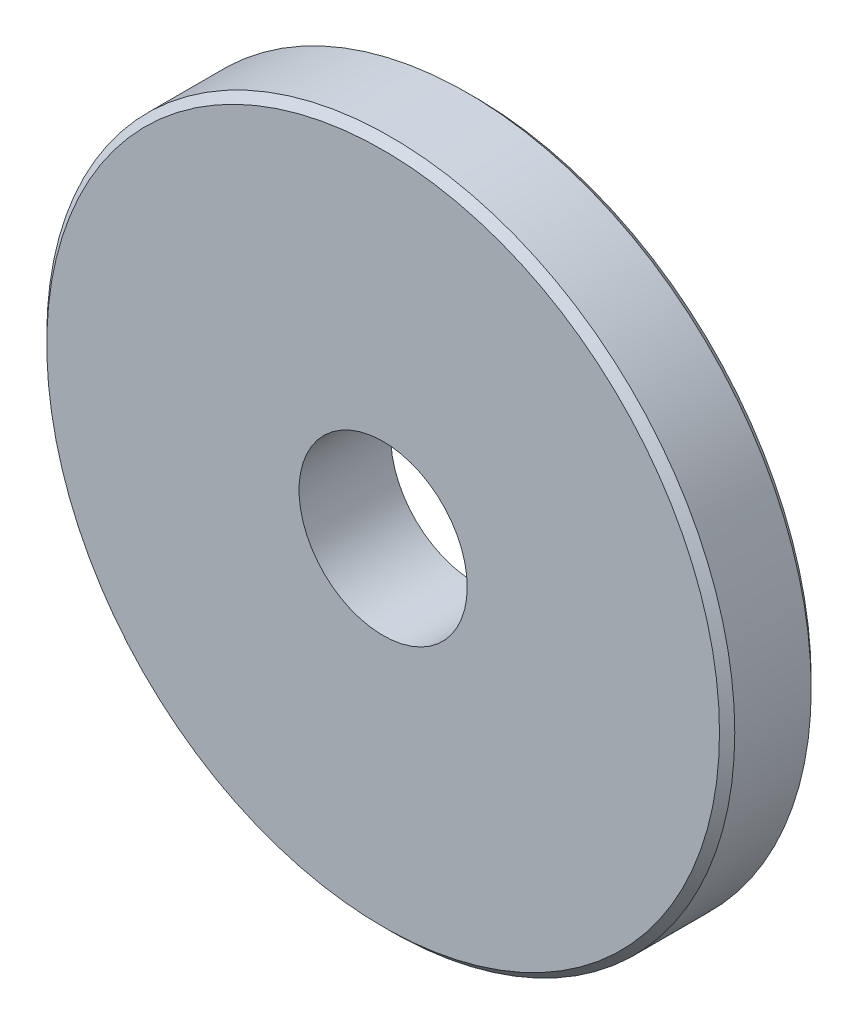
from build123d import *

# Parameters (mm, degrees)
SKETCH_1_R      = 22.5
SKETCH_1_R_2    = 5.5
EXTRUDE_1_DEPTH = 6
CHAMFER_1_SIZE  = 0.5


with BuildPart() as part:
    # 草图1 → 凸台-拉伸1 (new body)
    with BuildSketch(Plane.XY):
        Circle(SKETCH_1_R)
        Circle(SKETCH_1_R_2, mode=Mode.SUBTRACT)
    extrude(amount=EXTRUDE_1_DEPTH)

    # 倒角1
    chamfer_1_edges = [part.edges().sort_by_distance(p)[0] for p in [
        (-22.5, 0, 0),
        (-22.5, 0, 6),
    ]]
    chamfer(chamfer_1_edges, length=CHAMFER_1_SIZE)


solid = part.part
